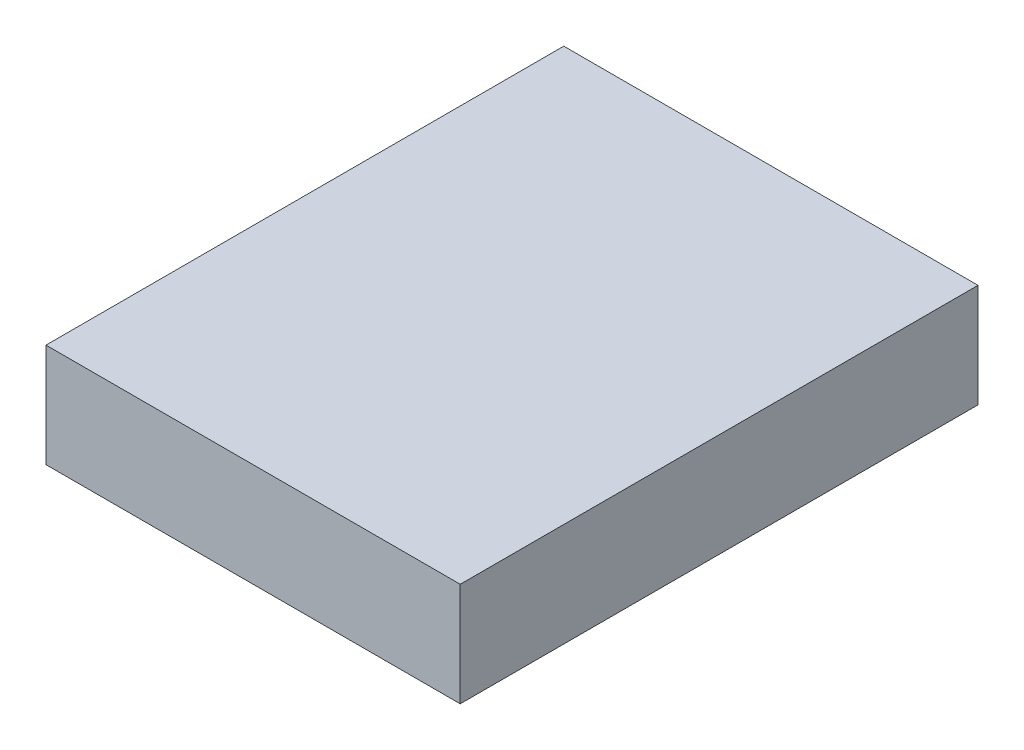
from build123d import *

# Parameters (mm, degrees)
SKETCH1_W      = 48
SKETCH1_H      = 60
EXTRUDE1_DEPTH = 6


with BuildPart() as part:
    # Sketch1 → Extrude1 (new, symmetric)
    with BuildSketch(Plane(origin=(0, 0, 0), x_dir=(1, 0, 0), z_dir=(0, 1, 0))):
        Rectangle(SKETCH1_W, SKETCH1_H)
    extrude(amount=EXTRUDE1_DEPTH, both=True)


solid = part.part
